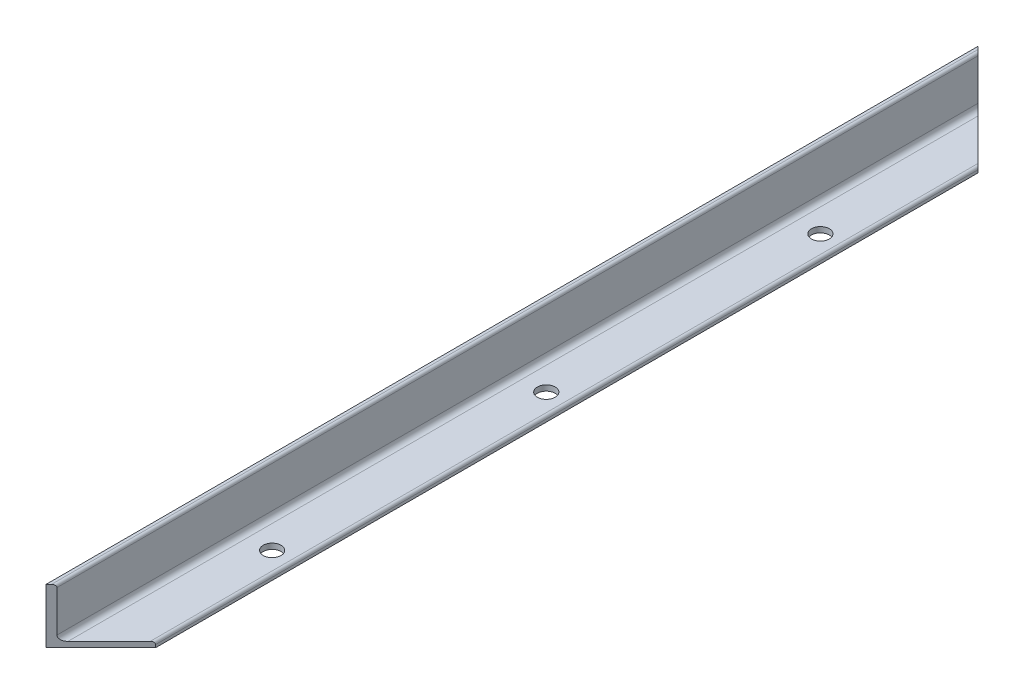
from build123d import *

# Parameters (mm, degrees)
BOSS_EXTRUDE1_DEPTH     = 680
CUT_EXTRUDE1_DEPTH      = 683.126088051
CUT_EXTRUDE1_DEPTH_BACK = 683.126088051
SKETCH3_R               = 6.5
CUT_EXTRUDE2_DEPTH      = 10


with BuildPart() as part:
    # Sketch1 → Boss-Extrude1 (new body)
    with BuildSketch(Plane.XY):
        with BuildLine():
            Line((0, 40), (0, 0))
            Line((0, 0), (40, 0))
            Line((40, 0), (40, 2))
            ThreePointArc((40, 2), (39.414213562, 3.414213562), (38, 4))
            Line((38, 4), (8, 4))
            ThreePointArc((8, 4), (5.171572875, 5.171572875), (4, 8))
            Line((4, 8), (4, 38))
            ThreePointArc((4, 38), (3.414213562, 39.414213562), (2, 40))
            Line((2, 40), (0, 40))
        make_face()
    extrude(amount=BOSS_EXTRUDE1_DEPTH)

    # Sketch2 → Cut-Extrude1 (cut, two sides: drawn at the far end of the back side and taken through both)
    with BuildSketch(Plane(origin=(0, 4, 0), x_dir=(1, 0, 0), z_dir=(0, 1, 0)).offset(-CUT_EXTRUDE1_DEPTH_BACK)):
        Polygon((0, 0), (40, -40), (40, 0), align=None)
        Polygon((0, -680), (40, -680), (40, -640), align=None)
    extrude(amount=CUT_EXTRUDE1_DEPTH + CUT_EXTRUDE1_DEPTH_BACK, mode=Mode.SUBTRACT)

    # Sketch3 → Cut-Extrude2 (cut)
    with BuildSketch(Plane(origin=(0, 4, 0), x_dir=(1, 0, 0), z_dir=(0, 1, 0))):
        with Locations(Location((25, -140, 0), (0, 0, 180))):
            Circle(SKETCH3_R)
        with Locations(Location((25, -340, 0), (0, 0, 180))):
            Circle(SKETCH3_R)
        with Locations(Location((25, -540, 0), (0, 0, 180))):
            Circle(SKETCH3_R)
    extrude(amount=-CUT_EXTRUDE2_DEPTH, mode=Mode.SUBTRACT)


solid = part.part
